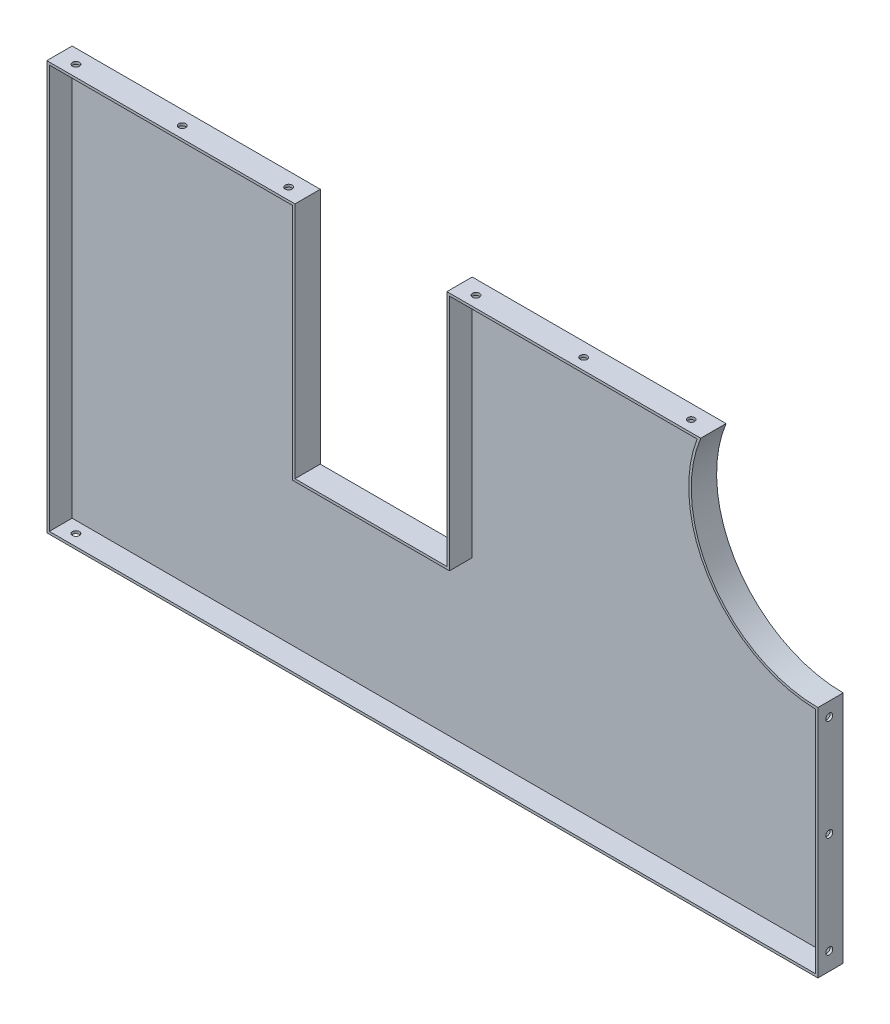
from build123d import *

# Parameters (mm, degrees)
EXTRUDE_1_DEPTH          = 20
SHELL_1_T                = -2
CUT_EXTRUDE_1_DEPTH      = 338
CUT_EXTRUDE_1_DEPTH_BACK = 10
SKETCH_2_R               = 2.75
SKETCH_3_R               = 2.75
CUT_EXTRUDE_2_DEPTH      = 10
SKETCH_4_R               = 2.75
CUT_EXTRUDE_3_DEPTH      = 10


with BuildPart() as part:
    # 草图1 → 凸台-拉伸1 (new body)
    with BuildSketch(Plane.XY):
        with BuildLine():
            Line((0, 0), (609, 0))
            Line((609, 0), (609, 185))
            ThreePointArc((609, 185), (525.933761371, 229.322356372), (516.501351361, 323))
            Line((516.501351361, 323), (316, 323))
            Line((316, 323), (316, 135))
            Line((316, 135), (196, 135))
            Line((196, 135), (196, 323))
            Line((196, 323), (0, 323))
            Line((0, 323), (0, 0))
        make_face()
    extrude(amount=EXTRUDE_1_DEPTH)

    # 抽壳1
    shell_1_openings = [part.faces().sort_by_distance(p)[0] for p in [
        (304.5, 6.893547708, 20),
    ]]
    offset(amount=SHELL_1_T, openings=shell_1_openings, kind=Kind.INTERSECTION)

    # 草图2 → 切除-拉伸1 (cut, two sides: drawn at the far end of the back side and taken through both)
    with BuildSketch(Plane(origin=(0, 2, 0), x_dir=(1, 0, 0), z_dir=(0, 1, 0)).offset(-CUT_EXTRUDE_1_DEPTH_BACK)):
        with Locations(Location((14, -11, 0), (0, 0, 90))):
            Circle(SKETCH_2_R)
    extrude(amount=CUT_EXTRUDE_1_DEPTH + CUT_EXTRUDE_1_DEPTH_BACK, mode=Mode.SUBTRACT)

    # 草图3 → 切除-拉伸2 (cut)
    with BuildSketch(Plane.XZ.offset(-321)):
        with Locations(Location((98, 11, 0), (0, 0, 270))):
            Circle(SKETCH_3_R)
        with Locations(Location((182, 11, 0), (0, 0, 270))):
            Circle(SKETCH_3_R)
        with Locations(Location((330, 11, 0), (0, 0, 270))):
            Circle(SKETCH_3_R)
        with Locations(Location((415, 11, 0), (0, 0, 270))):
            Circle(SKETCH_3_R)
        with Locations(Location((500, 11, 0), (0, 0, 270))):
            Circle(SKETCH_3_R)
    extrude(amount=-CUT_EXTRUDE_2_DEPTH, mode=Mode.SUBTRACT)

    # 草图4 → 切除-拉伸3 (cut)
    with BuildSketch(Plane.ZY.offset(-607)):
        with Locations((11, 14)):
            Circle(SKETCH_4_R)
        with Locations((11, 94)):
            Circle(SKETCH_4_R)
        with Locations((11, 174)):
            Circle(SKETCH_4_R)
    extrude(amount=-CUT_EXTRUDE_3_DEPTH, mode=Mode.SUBTRACT)


solid = part.part
